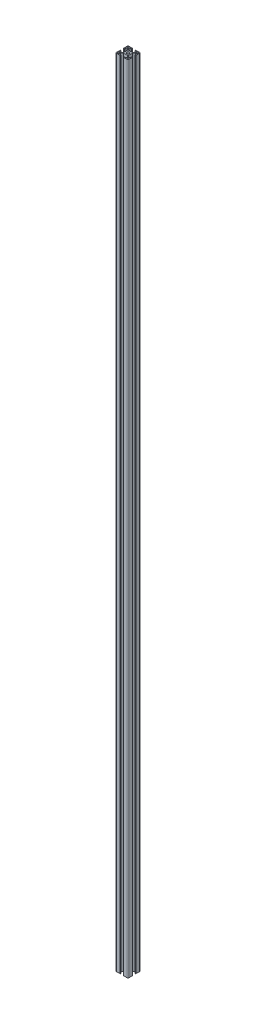
SolidWorks part; units mm, degrees
ref_plane "前视基准面" through (0, 0, 0) normal (0, 0, 1) x (1, 0, 0)
ref_plane "上视基准面" through (0, 0, 0) normal (0, 1, 0) x (1, 0, 0)
ref_plane "右视基准面" through (0, 0, 0) normal (1, 0, 0) x (0, 0, -1)
sketch "草图1" plane through (0, 0, 0) normal (0, 1, 0) x (1, 0, 0)
  line L44 (6.75, -28) -> (11, -28)
  line L45 (11, -28) -> (11, -30)
  line L46 (11, -30) -> (2, -30)
  line L47 (0, -28) -> (0, -19)
  line L48 (0, -19) -> (2, -19)
  line L49 (2, -19) -> (2, -23.25)
  line L50 (28, -30) -> (19, -30)
  line L51 (19, -30) -> (19, -28)
  line L52 (23.25, -28) -> (23.25, -24.6642)
  line L53 (19, -28) -> (23.25, -28)
  line L54 (30, -19) -> (30, -28)
  line L55 (28, -19) -> (30, -19)
  line L56 (28, -23.25) -> (28, -19)
  line L57 (24.6642, -23.25) -> (28, -23.25)
  line L58 (21, -19.5858) -> (24.6642, -23.25)
  line L59 (23.25, -24.6642) -> (19.5858, -21)
  line L60 (6.75, -24.6642) -> (6.75, -28)
  line L61 (2, -23.25) -> (5.3358, -23.25)
  line L62 (5.3358, -23.25) -> (9, -19.5858)
  line L63 (10.4142, -21) -> (6.75, -24.6642)
  line L64 (19.5858, -21) -> (10.4142, -21)
  line L65 (9, -19.5858) -> (9, -10.4142)
  line L66 (21, -10.4142) -> (21, -19.5858)
  line L67 (30, -11) -> (28, -11)
  line L68 (28, -11) -> (28, -6.75)
  line L69 (28, -6.75) -> (24.6642, -6.75)
  line L70 (24.6642, -6.75) -> (21, -10.4142)
  line L71 (19.5858, -9) -> (23.25, -5.3358)
  line L72 (10.4142, -9) -> (19.5858, -9)
  line L73 (6.75, -5.3358) -> (10.4142, -9)
  line L74 (9, -10.4142) -> (5.3358, -6.75)
  line L75 (2, -11) -> (0, -11)
  line L76 (2, -6.75) -> (2, -11)
  line L77 (5.3358, -6.75) -> (2, -6.75)
  line L78 (6.75, -2) -> (6.75, -5.3358)
  line L79 (23.25, -5.3358) -> (23.25, -2)
  line L80 (23.25, -2) -> (19, -2)
  line L81 (19, -2) -> (19, 0)
  line L82 (11, 0) -> (11, -2)
  line L83 (11, -2) -> (6.75, -2)
  line L84 (30, -2) -> (30, -11)
  line L85 (19, 0) -> (28, 0)
  line L86 (2, 0) -> (11, 0)
  line L87 (0, -11) -> (0, -2)
  line L88 (0, -15) -> (30, -15) construction
  line L89 (15, -30) -> (15, 0) construction
  line L90 (0, 0) -> (30, -30) construction
  line L91 (0, -30) -> (30, 0) construction
  arc A9 (0, -28) -> (2, -30) centre (2, -28) ccw
  circle A10 centre (3.375, -26.625) radius 2.1
  circle A11 centre (26.625, -26.625) radius 2.1
  arc A12 (28, -30) -> (30, -28) centre (28, -28) ccw
  circle A13 centre (15, -15) radius 3.4
  circle A14 centre (3.375, -3.375) radius 2.1
  circle A15 centre (26.625, -3.375) radius 2.1
  arc A16 (30, -2) -> (28, 0) centre (28, -2) ccw
  arc A17 (2, 0) -> (0, -2) centre (2, -2) ccw
  dimension "D2" = 15
  dimension "D5" = 6.8
  dimension "D8" = 6
  dimension "D11" = 23.25
  dimension "D12" = 3.375
  dimension "D13" = 23.25
  dimension "D14" = 4.2
  dimension "D15" = 2
  dimension "D16" = 2
  dimension "D23" = 2
  dimension "D24" = 2
  dimension "D1" = 15
  dimension "D3" = 45
  dimension "D4" = 45
  dimension "D6" = 30
  dimension "D7" = 30
  dimension "D9" = 12
  dimension "D10" = 3.375
  dimension "D17" = 11
  dimension "D18" = 8
  dimension "D19" = 2
  dimension "D20" = 2
  dimension "D21" = 11
  dimension "D22" = 8
  dimension "D25" = 2
  dimension "D26" = 2
  dimension "D27" = 6.75
  dimension "D28" = 16.5
  dimension "D29" = 6.75
  dimension "D30" = 16.5
  dimension "D31" = 12
  dimension "D32" = 6
  dimension "D33" = 2
  dimension "D34" = 1
  dimension "D35" = 2
  dimension "D36" = 1
extrude "拉伸1" add sketch "草图1" along normal blind 1940
hole_wizard "打孔尺寸根据内六角圆柱头螺钉的类型1" positions "草图3" profile "草图2" counterbore size "M6" standard "GB" end condition through all
sketch "草图3" plane through (0, 0, 0) normal (-1, 0, 0) x (0, 0, 1)
  line L0 (0, 1940) -> (0, 0) construction
  line L1 (2, 1940) -> (11, 1940) construction
  line L2 (10.4142, 0) -> (19.5858, 0) construction
  line L3 (15, 1940) -> (15, 0) construction
  line L4 (10.4142, 1940) -> (19.5858, 1940) construction
  point P3 (15, 70)
  point P9 (15, 1870)
  point P26 (15, 1270)
  point P28 (15, 670)
  dimension "D1" = 15
  dimension "D2" = 70
  dimension "D3" = 70
  dimension "D4" = 600
  dimension "D5" = 600
sketch "草图2" plane through (0, 70, 15) normal (0, 1, 0) x (0, 0, 1)
  line L0 (0, 0) -> (0, 30)
  line L1 (0, 30) -> (3.3, 30)
  line L3 (3.3, 30) -> (3.3, 9)
  line L4 (3.3, 9) -> (5.5, 9)
  line L5 (5.5, 9) -> (5.5, 0)
  line L7 (5.5, 0) -> (0, 0)
  line L11 (0, -6.35) -> (0, 107.95) construction
  dimension "通孔孔直径" = 6.6
  dimension "通孔孔深度" = 30
  dimension "柱形沉头孔直径" = 11
  dimension "柱形沉头孔深度" = 9
